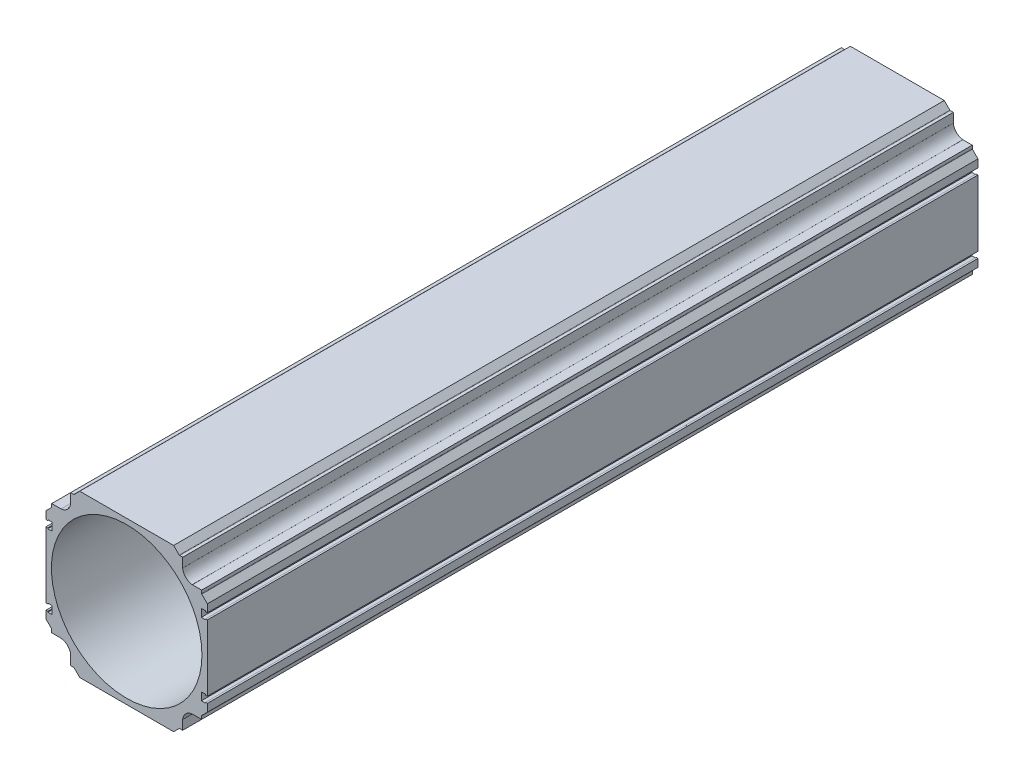
from build123d import *

# Parameters (mm, degrees)
SKETCH1_R           = 62.5
BOSS_EXTRUDE1_DEPTH = 640


with BuildPart() as part:
    # Sketch1 → Boss-Extrude1 (new body)
    with BuildSketch(Plane.XY):
        with BuildLine():
            add(Edge.make_bspline(
                [(60.749353033, -32.575), (60.249353033, -32.575), (59.749353033, -32.575), (59.249353033, -32.575)],
                knots=[0, 0, 0, 0, 1, 1, 1, 1], degree=3))
            add(Edge.make_bspline(
                [(59.249353033, -32.575), (59.249353033, -32.8), (59.249353033, -33.025), (59.249353033, -33.25)],
                knots=[0, 0, 0, 0, 1, 1, 1, 1], degree=3))
            add(Edge.make_bspline(
                [(59.249353033, -33.25), (58.082686367, -33.25), (56.9160197, -33.25), (55.749353033, -33.25)],
                knots=[0, 0, 0, 0, 1, 1, 1, 1], degree=3))
            add(Edge.make_bspline(
                [(55.749353033, -33.25), (55.749353033, -31.083333333), (55.749353033, -28.916666667), (55.749353033, -26.75)],
                knots=[0, 0, 0, 0, 1, 1, 1, 1], degree=3))
            add(Edge.make_bspline(
                [(55.749353033, -26.75), (56.9160197, -26.75), (58.082686367, -26.75), (59.249353033, -26.75)],
                knots=[0, 0, 0, 0, 1, 1, 1, 1], degree=3))
            add(Edge.make_bspline(
                [(59.249353033, -26.75), (59.249353033, -26.975), (59.249353033, -27.2), (59.249353033, -27.425)],
                knots=[0, 0, 0, 0, 1, 1, 1, 1], degree=3))
            add(Edge.make_bspline(
                [(59.249353033, -27.425), (59.749353033, -27.425), (60.249353033, -27.425), (60.749353033, -27.425)],
                knots=[0, 0, 0, 0, 1, 1, 1, 1], degree=3))
            add(Edge.make_bspline(
                [(60.749353033, -27.425), (60.749353033, -9.141666667), (60.749353033, 9.141666667), (60.749353033, 27.425)],
                knots=[0, 0, 0, 0, 1, 1, 1, 1], degree=3))
            add(Edge.make_bspline(
                [(60.749353033, 27.425), (60.249353033, 27.425), (59.749353033, 27.425), (59.249353033, 27.425)],
                knots=[0, 0, 0, 0, 1, 1, 1, 1], degree=3))
            add(Edge.make_bspline(
                [(59.249353033, 27.425), (59.249353033, 27.2), (59.249353033, 26.975), (59.249353033, 26.75)],
                knots=[0, 0, 0, 0, 1, 1, 1, 1], degree=3))
            add(Edge.make_bspline(
                [(59.249353033, 26.75), (58.082686367, 26.75), (56.9160197, 26.75), (55.749353033, 26.75)],
                knots=[0, 0, 0, 0, 1, 1, 1, 1], degree=3))
            add(Edge.make_bspline(
                [(55.749353033, 26.75), (55.749353033, 28.916666667), (55.749353033, 31.083333333), (55.749353033, 33.25)],
                knots=[0, 0, 0, 0, 1, 1, 1, 1], degree=3))
            add(Edge.make_bspline(
                [(55.749353033, 33.25), (56.9160197, 33.25), (58.082686367, 33.25), (59.249353033, 33.25)],
                knots=[0, 0, 0, 0, 1, 1, 1, 1], degree=3))
            add(Edge.make_bspline(
                [(59.249353033, 33.25), (59.249353033, 33.025), (59.249353033, 32.8), (59.249353033, 32.575)],
                knots=[0, 0, 0, 0, 1, 1, 1, 1], degree=3))
            add(Edge.make_bspline(
                [(59.249353033, 32.575), (59.749353033, 32.575), (60.249353033, 32.575), (60.749353033, 32.575)],
                knots=[0, 0, 0, 0, 1, 1, 1, 1], degree=3))
            add(Edge.make_bspline(
                [(60.749353033, 32.575), (60.749353033, 34.716666667), (60.749353033, 36.858333333), (60.749353033, 39)],
                knots=[0, 0, 0, 0, 1, 1, 1, 1], degree=3))
            add(Edge.make_bspline(
                [(60.749353033, 39), (59.212501903, 40.53685113), (57.675650773, 42.07370226), (56.138799643, 43.610553391)],
                knots=[0, 0, 0, 0, 1, 1, 1, 1], degree=3))
            add(Edge.make_bspline(
                [(56.138799643, 43.610553391), (56.045301702, 43.704051331), (55.992353033, 43.831118371), (55.992353033, 43.964106781)],
                knots=[0, 0, 0, 0, 1, 1, 1, 1], degree=3))
            add(Edge.make_bspline(
                [(55.992353033, 43.964106781), (55.992353033, 44.809404521), (55.992353033, 45.65470226), (55.992353033, 46.5)],
                knots=[0, 0, 0, 0, 1, 1, 1, 1], degree=3))
            add(Edge.make_bspline(
                [(55.992353033, 46.5), (53.411353033, 46.5), (50.830353033, 46.5), (48.249353033, 46.5)],
                knots=[0, 0, 0, 0, 1, 1, 1, 1], degree=3))
            add(Edge.make_bspline(
                [(48.249353033, 46.5), (48.244134488, 46.505218546), (48.238915942, 46.510437092), (48.233697396, 46.515655637)],
                knots=[0, 0, 0, 0, 1, 1, 1, 1], degree=3))
            add(Edge.make_bspline(
                [(48.233697396, 46.515655637), (44.124880551, 46.765378477), (40.514910931, 50.372575428), (40.265008671, 54.484344363)],
                knots=[0, 0, 0, 0, 1, 1, 1, 1], degree=3))
            add(Edge.make_bspline(
                [(40.265008671, 54.484344363), (40.259790125, 54.489562908), (40.254571579, 54.494781454), (40.249353033, 54.5)],
                knots=[0, 0, 0, 0, 1, 1, 1, 1], degree=3))
            add(Edge.make_bspline(
                [(40.249353033, 54.5), (40.249353033, 57.081), (40.249353033, 59.662), (40.249353033, 62.243)],
                knots=[0, 0, 0, 0, 1, 1, 1, 1], degree=3))
            add(Edge.make_bspline(
                [(40.249353033, 62.243), (39.404055294, 62.243), (38.558757554, 62.243), (37.713459815, 62.243)],
                knots=[0, 0, 0, 0, 1, 1, 1, 1], degree=3))
            add(Edge.make_bspline(
                [(37.713459815, 62.243), (37.581233759, 62.243), (37.45394343, 62.295409603), (37.359906424, 62.389446609)],
                knots=[0, 0, 0, 0, 1, 1, 1, 1], degree=3))
            add(Edge.make_bspline(
                [(37.359906424, 62.389446609), (35.823055294, 63.92629774), (34.286204164, 65.46314887), (32.749353033, 67)],
                knots=[0, 0, 0, 0, 1, 1, 1, 1], degree=3))
            add(Edge.make_bspline(
                [(32.749353033, 67), (6.749353033, 67), (-19.250646967, 67), (-45.250646967, 67)],
                knots=[0, 0, 0, 0, 1, 1, 1, 1], degree=3))
            add(Edge.make_bspline(
                [(-45.250646967, 67), (-46.787498097, 65.46314887), (-48.324349227, 63.92629774), (-49.861200357, 62.389446609)],
                knots=[0, 0, 0, 0, 1, 1, 1, 1], degree=3))
            add(Edge.make_bspline(
                [(-49.861200357, 62.389446609), (-49.954698298, 62.295948669), (-50.081765338, 62.243), (-50.214753748, 62.243)],
                knots=[0, 0, 0, 0, 1, 1, 1, 1], degree=3))
            add(Edge.make_bspline(
                [(-50.214753748, 62.243), (-51.060051487, 62.243), (-51.905349227, 62.243), (-52.750646967, 62.243)],
                knots=[0, 0, 0, 0, 1, 1, 1, 1], degree=3))
            add(Edge.make_bspline(
                [(-52.750646967, 62.243), (-52.750646967, 59.662), (-52.750646967, 57.081), (-52.750646967, 54.5)],
                knots=[0, 0, 0, 0, 1, 1, 1, 1], degree=3))
            add(Edge.make_bspline(
                [(-52.750646967, 54.5), (-52.755865512, 54.494781454), (-52.761084058, 54.489562908), (-52.766302604, 54.484344363)],
                knots=[0, 0, 0, 0, 1, 1, 1, 1], degree=3))
            add(Edge.make_bspline(
                [(-52.766302604, 54.484344363), (-53.016025444, 50.375527517), (-56.623222395, 46.765557897), (-60.734991329, 46.515655637)],
                knots=[0, 0, 0, 0, 1, 1, 1, 1], degree=3))
            add(Edge.make_bspline(
                [(-60.734991329, 46.515655637), (-60.740209875, 46.510437092), (-60.745428421, 46.505218546), (-60.750646967, 46.5)],
                knots=[0, 0, 0, 0, 1, 1, 1, 1], degree=3))
            add(Edge.make_bspline(
                [(-60.750646967, 46.5), (-63.331646967, 46.5), (-65.912646967, 46.5), (-68.493646967, 46.5)],
                knots=[0, 0, 0, 0, 1, 1, 1, 1], degree=3))
            add(Edge.make_bspline(
                [(-68.493646967, 46.5), (-68.493646967, 45.65470226), (-68.493646967, 44.809404521), (-68.493646967, 43.964106781)],
                knots=[0, 0, 0, 0, 1, 1, 1, 1], degree=3))
            add(Edge.make_bspline(
                [(-68.493646967, 43.964106781), (-68.493646967, 43.831880726), (-68.54605657, 43.704590397), (-68.640093576, 43.610553391)],
                knots=[0, 0, 0, 0, 1, 1, 1, 1], degree=3))
            add(Edge.make_bspline(
                [(-68.640093576, 43.610553391), (-70.176944706, 42.07370226), (-71.713795836, 40.53685113), (-73.250646967, 39)],
                knots=[0, 0, 0, 0, 1, 1, 1, 1], degree=3))
            add(Edge.make_bspline(
                [(-73.250646967, 39), (-73.250646967, 36.858333333), (-73.250646967, 34.716666667), (-73.250646967, 32.575)],
                knots=[0, 0, 0, 0, 1, 1, 1, 1], degree=3))
            add(Edge.make_bspline(
                [(-73.250646967, 32.575), (-72.750646967, 32.575), (-72.250646967, 32.575), (-71.750646967, 32.575)],
                knots=[0, 0, 0, 0, 1, 1, 1, 1], degree=3))
            add(Edge.make_bspline(
                [(-71.750646967, 32.575), (-71.750646967, 32.8), (-71.750646967, 33.025), (-71.750646967, 33.25)],
                knots=[0, 0, 0, 0, 1, 1, 1, 1], degree=3))
            add(Edge.make_bspline(
                [(-71.750646967, 33.25), (-70.5839803, 33.25), (-69.417313633, 33.25), (-68.250646967, 33.25)],
                knots=[0, 0, 0, 0, 1, 1, 1, 1], degree=3))
            add(Edge.make_bspline(
                [(-68.250646967, 33.25), (-68.250646967, 31.083333333), (-68.250646967, 28.916666667), (-68.250646967, 26.75)],
                knots=[0, 0, 0, 0, 1, 1, 1, 1], degree=3))
            add(Edge.make_bspline(
                [(-68.250646967, 26.75), (-69.417313633, 26.75), (-70.5839803, 26.75), (-71.750646967, 26.75)],
                knots=[0, 0, 0, 0, 1, 1, 1, 1], degree=3))
            add(Edge.make_bspline(
                [(-71.750646967, 26.75), (-71.750646967, 26.975), (-71.750646967, 27.2), (-71.750646967, 27.425)],
                knots=[0, 0, 0, 0, 1, 1, 1, 1], degree=3))
            add(Edge.make_bspline(
                [(-71.750646967, 27.425), (-72.250646967, 27.425), (-72.750646967, 27.425), (-73.250646967, 27.425)],
                knots=[0, 0, 0, 0, 1, 1, 1, 1], degree=3))
            add(Edge.make_bspline(
                [(-73.250646967, 27.425), (-73.250646967, 9.141666667), (-73.250646967, -9.141666667), (-73.250646967, -27.425)],
                knots=[0, 0, 0, 0, 1, 1, 1, 1], degree=3))
            add(Edge.make_bspline(
                [(-73.250646967, -27.425), (-72.750646967, -27.425), (-72.250646967, -27.425), (-71.750646967, -27.425)],
                knots=[0, 0, 0, 0, 1, 1, 1, 1], degree=3))
            add(Edge.make_bspline(
                [(-71.750646967, -27.425), (-71.750646967, -27.2), (-71.750646967, -26.975), (-71.750646967, -26.75)],
                knots=[0, 0, 0, 0, 1, 1, 1, 1], degree=3))
            add(Edge.make_bspline(
                [(-71.750646967, -26.75), (-70.5839803, -26.75), (-69.417313633, -26.75), (-68.250646967, -26.75)],
                knots=[0, 0, 0, 0, 1, 1, 1, 1], degree=3))
            add(Edge.make_bspline(
                [(-68.250646967, -26.75), (-68.250646967, -28.916666667), (-68.250646967, -31.083333333), (-68.250646967, -33.25)],
                knots=[0, 0, 0, 0, 1, 1, 1, 1], degree=3))
            add(Edge.make_bspline(
                [(-68.250646967, -33.25), (-69.417313633, -33.25), (-70.5839803, -33.25), (-71.750646967, -33.25)],
                knots=[0, 0, 0, 0, 1, 1, 1, 1], degree=3))
            add(Edge.make_bspline(
                [(-71.750646967, -33.25), (-71.750646967, -33.025), (-71.750646967, -32.8), (-71.750646967, -32.575)],
                knots=[0, 0, 0, 0, 1, 1, 1, 1], degree=3))
            add(Edge.make_bspline(
                [(-71.750646967, -32.575), (-72.250646967, -32.575), (-72.750646967, -32.575), (-73.250646967, -32.575)],
                knots=[0, 0, 0, 0, 1, 1, 1, 1], degree=3))
            add(Edge.make_bspline(
                [(-73.250646967, -32.575), (-73.250646967, -34.716666667), (-73.250646967, -36.858333333), (-73.250646967, -39)],
                knots=[0, 0, 0, 0, 1, 1, 1, 1], degree=3))
            add(Edge.make_bspline(
                [(-73.250646967, -39), (-71.713795836, -40.53685113), (-70.176944706, -42.07370226), (-68.640093576, -43.610553391)],
                knots=[0, 0, 0, 0, 1, 1, 1, 1], degree=3))
            add(Edge.make_bspline(
                [(-68.640093576, -43.610553391), (-68.546595635, -43.704051331), (-68.493646967, -43.831118371), (-68.493646967, -43.964106781)],
                knots=[0, 0, 0, 0, 1, 1, 1, 1], degree=3))
            add(Edge.make_bspline(
                [(-68.493646967, -43.964106781), (-68.493646967, -44.809404521), (-68.493646967, -45.65470226), (-68.493646967, -46.5)],
                knots=[0, 0, 0, 0, 1, 1, 1, 1], degree=3))
            add(Edge.make_bspline(
                [(-68.493646967, -46.5), (-65.912646967, -46.5), (-63.331646967, -46.5), (-60.750646967, -46.5)],
                knots=[0, 0, 0, 0, 1, 1, 1, 1], degree=3))
            add(Edge.make_bspline(
                [(-60.750646967, -46.5), (-60.745428421, -46.505218546), (-60.740209875, -46.510437092), (-60.734991329, -46.515655637)],
                knots=[0, 0, 0, 0, 1, 1, 1, 1], degree=3))
            add(Edge.make_bspline(
                [(-60.734991329, -46.515655637), (-56.626174484, -46.765378477), (-53.016204864, -50.372575428), (-52.766302604, -54.484344363)],
                knots=[0, 0, 0, 0, 1, 1, 1, 1], degree=3))
            add(Edge.make_bspline(
                [(-52.766302604, -54.484344363), (-52.761084058, -54.489562908), (-52.755865512, -54.494781454), (-52.750646967, -54.5)],
                knots=[0, 0, 0, 0, 1, 1, 1, 1], degree=3))
            add(Edge.make_bspline(
                [(-52.750646967, -54.5), (-52.750646967, -57.081), (-52.750646967, -59.662), (-52.750646967, -62.243)],
                knots=[0, 0, 0, 0, 1, 1, 1, 1], degree=3))
            add(Edge.make_bspline(
                [(-52.750646967, -62.243), (-51.905349227, -62.243), (-51.060051487, -62.243), (-50.214753748, -62.243)],
                knots=[0, 0, 0, 0, 1, 1, 1, 1], degree=3))
            add(Edge.make_bspline(
                [(-50.214753748, -62.243), (-50.082527692, -62.243), (-49.955237364, -62.295409603), (-49.861200357, -62.389446609)],
                knots=[0, 0, 0, 0, 1, 1, 1, 1], degree=3))
            add(Edge.make_bspline(
                [(-49.861200357, -62.389446609), (-48.324349227, -63.92629774), (-46.787498097, -65.46314887), (-45.250646967, -67)],
                knots=[0, 0, 0, 0, 1, 1, 1, 1], degree=3))
            add(Edge.make_bspline(
                [(-45.250646967, -67), (-19.250646967, -67), (6.749353033, -67), (32.749353033, -67)],
                knots=[0, 0, 0, 0, 1, 1, 1, 1], degree=3))
            add(Edge.make_bspline(
                [(32.749353033, -67), (34.286204164, -65.46314887), (35.823055294, -63.92629774), (37.359906424, -62.389446609)],
                knots=[0, 0, 0, 0, 1, 1, 1, 1], degree=3))
            add(Edge.make_bspline(
                [(37.359906424, -62.389446609), (37.453404365, -62.295948669), (37.580471405, -62.243), (37.713459815, -62.243)],
                knots=[0, 0, 0, 0, 1, 1, 1, 1], degree=3))
            add(Edge.make_bspline(
                [(37.713459815, -62.243), (38.558757554, -62.243), (39.404055294, -62.243), (40.249353033, -62.243)],
                knots=[0, 0, 0, 0, 1, 1, 1, 1], degree=3))
            add(Edge.make_bspline(
                [(40.249353033, -62.243), (40.249353033, -59.662), (40.249353033, -57.081), (40.249353033, -54.5)],
                knots=[0, 0, 0, 0, 1, 1, 1, 1], degree=3))
            add(Edge.make_bspline(
                [(40.249353033, -54.5), (40.254571579, -54.494781454), (40.259790125, -54.489562908), (40.265008671, -54.484344363)],
                knots=[0, 0, 0, 0, 1, 1, 1, 1], degree=3))
            add(Edge.make_bspline(
                [(40.265008671, -54.484344363), (40.514731511, -50.375527518), (44.121928461, -46.765557897), (48.233697396, -46.515655637)],
                knots=[0, 0, 0, 0, 1, 1, 1, 1], degree=3))
            add(Edge.make_bspline(
                [(48.233697396, -46.515655637), (48.238915942, -46.510437092), (48.244134488, -46.505218546), (48.249353033, -46.5)],
                knots=[0, 0, 0, 0, 1, 1, 1, 1], degree=3))
            add(Edge.make_bspline(
                [(48.249353033, -46.5), (50.830353033, -46.5), (53.411353033, -46.5), (55.992353033, -46.5)],
                knots=[0, 0, 0, 0, 1, 1, 1, 1], degree=3))
            add(Edge.make_bspline(
                [(55.992353033, -46.5), (55.992353033, -45.65470226), (55.992353033, -44.809404521), (55.992353033, -43.964106781)],
                knots=[0, 0, 0, 0, 1, 1, 1, 1], degree=3))
            add(Edge.make_bspline(
                [(55.992353033, -43.964106781), (55.992353033, -43.831880726), (56.044762636, -43.704590397), (56.138799643, -43.610553391)],
                knots=[0, 0, 0, 0, 1, 1, 1, 1], degree=3))
            add(Edge.make_bspline(
                [(56.138799643, -43.610553391), (57.675650773, -42.07370226), (59.212501903, -40.53685113), (60.749353033, -39)],
                knots=[0, 0, 0, 0, 1, 1, 1, 1], degree=3))
            add(Edge.make_bspline(
                [(60.749353033, -39), (60.749353033, -36.858333333), (60.749353033, -34.716666667), (60.749353033, -32.575)],
                knots=[0, 0, 0, 0, 1, 1, 1, 1], degree=3))
        make_face()
        with Locations((-6.250646967, 0)):
            Circle(SKETCH1_R, mode=Mode.SUBTRACT)
    extrude(amount=BOSS_EXTRUDE1_DEPTH)


solid = part.part
